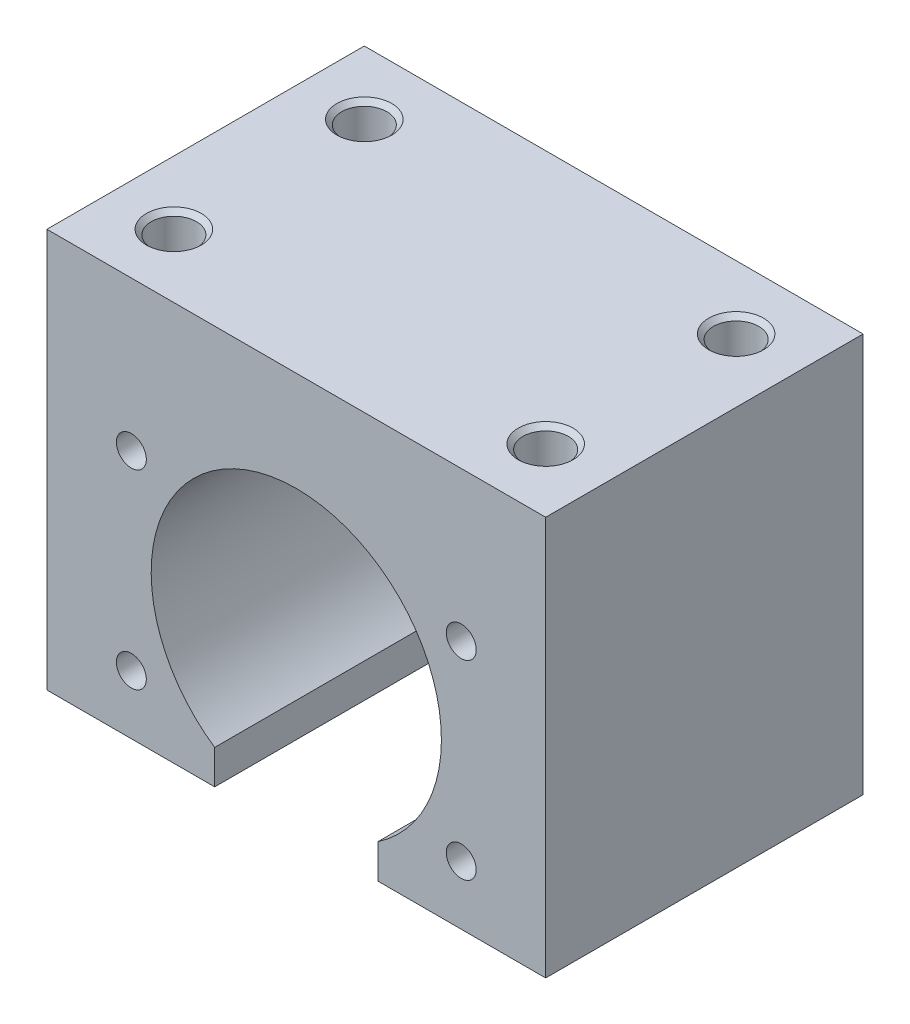
SolidWorks part; units mm, degrees
ref_plane "前视基准面" through (0, 0, 0) normal (0, 0, 1) x (1, 0, 0)
ref_plane "上视基准面" through (0, 0, 0) normal (0, 1, 0) x (1, 0, 0)
ref_plane "右视基准面" through (0, 0, 0) normal (1, 0, 0) x (0, 0, -1)
sketch "草图1" plane through (0, 0, 0) normal (0, 0, 1) x (1, 0, 0)
  line L0 (-27.5, 27) -> (27.5, 27)
  line L1 (27.5, 27) -> (27.5, -17)
  line L2 (27.5, -17) -> (9, -17)
  line L3 (9, -17) -> (9, -13.2288)
  line L4 (-27.5, 27) -> (-27.5, -17)
  line L5 (-27.5, -17) -> (-9, -17)
  line L6 (-9, -17) -> (-9, -13.2288)
  arc A0 (9, -13.2288) -> (-9, -13.2288) centre (0, 0) ccw
extrude "凸台-拉伸1" add sketch "草图1" along normal mid plane 35
hole_wizard "M4 螺纹孔1" positions "草图3" profile "草图2" tap size "M4" standard "GB"
sketch "草图3" plane through (0, 0, 17.5) normal (0, 0, 1) x (1, 0, 0)
  circle A0 centre (18.1865, 10.5) radius 2.25 construction
  circle A1 centre (18.1865, -10.5) radius 2.25 construction
  circle A2 centre (-18.1865, -10.5) radius 2.25 construction
  circle A3 centre (-18.1865, 10.5) radius 2.25 construction
  point P1 (18.1865, 10.5)
  point P5 (18.1865, -10.5)
  point P9 (-18.1865, -10.5)
  point P13 (-18.1865, 10.5)
cosmetic thread "孔螺蚊线1" parameters "D1"=6, "D2"=4
cosmetic thread "孔螺蚊线2" parameters "D1"=6, "D2"=4
cosmetic thread "孔螺蚊线3" parameters "D1"=6, "D2"=4
cosmetic thread "孔螺蚊线4" parameters "D1"=6, "D2"=4
sketch "草图2" plane through (18.1865, 10.5, 17.5) normal (1, 0, 0) x (0, -1, 0)
  line L0 (0, 0) -> (0, 10.4914)
  line L1 (0, 10.4914) -> (1.65, 9.5)
  line L2 (1.65, 9.5) -> (1.65, 0)
  line L5 (1.65, 0) -> (0, 0)
  line L10 (0, 10.4914) -> (-1.65, 9.5) construction
  line L11 (0, -6.35) -> (0, 107.95) construction
  dimension "螺纹孔钻头直径" = 3.3
  dimension "螺纹孔钻头深度" = 9.5
  dimension "导头角度" = 118
sketch "草图4" plane through (0, 27, 0) normal (0, 1, 0) x (1, 0, 0)
  line L0 (27.5, -17.5) -> (27.5, 17.5) construction
  line L1 (-20.5, -10.5) -> (20.5, -10.5)
  line L2 (-20.5, -10.5) -> (-20.5, 10.5)
  line L3 (-20.5, 10.5) -> (20.5, 10.5)
  line L4 (20.5, -10.5) -> (20.5, 10.5)
  line L5 (-20.5, -10.5) -> (20.5, 10.5) construction
  line L6 (-20.5, 10.5) -> (20.5, -10.5) construction
  line L7 (27.5, -17.5) -> (-27.5, -17.5) construction
  point P0 (0, 0)
  dimension "D1" = 7
  dimension "D2" = 7
hole_wizard "M6 螺纹孔1" positions "3D草图1" profile "草图5" tap size "M6" standard "GB"
sketch3d "3D草图1"
  point P0 (-20.5, 27, 10.5)
  point P3 (-20.5, 27, -10.5)
  point P6 (20.5, 27, -10.5)
  point P9 (20.5, 27, 10.5)
sketch "草图5" plane through (-20.5, 27, 10.5) normal (1, 0, 0) x (0, 0, 1)
  line L0 (0, 0) -> (0, 13.5022)
  line L1 (0, 13.5022) -> (2.5, 12)
  line L2 (2.5, 12) -> (2.5, 0.525)
  line L3 (2.5, 0.525) -> (3.025, 0)
  line L5 (3.025, 0) -> (0, 0)
  line L6 (-2.5, 0.525) -> (-3.025, 0) construction
  line L10 (0, 13.5022) -> (-2.5, 12) construction
  line L11 (0, -6.35) -> (0, 107.95) construction
  dimension "螺纹孔钻头直径" = 5
  dimension "螺纹孔钻头深度" = 12
  dimension "近端锥形沉头孔直径" = 6.05
  dimension "近端锥形沉头孔角度" = 90
  dimension "导头角度" = 118
cosmetic thread "孔螺蚊线5" parameters "D1"=8, "D2"=6
cosmetic thread "孔螺蚊线6" parameters "D1"=8, "D2"=6
cosmetic thread "孔螺蚊线7" parameters "D1"=8, "D2"=6
cosmetic thread "孔螺蚊线8" parameters "D1"=8, "D2"=6
equation "\"D3@草图1\"=\"D2@草图1\""
